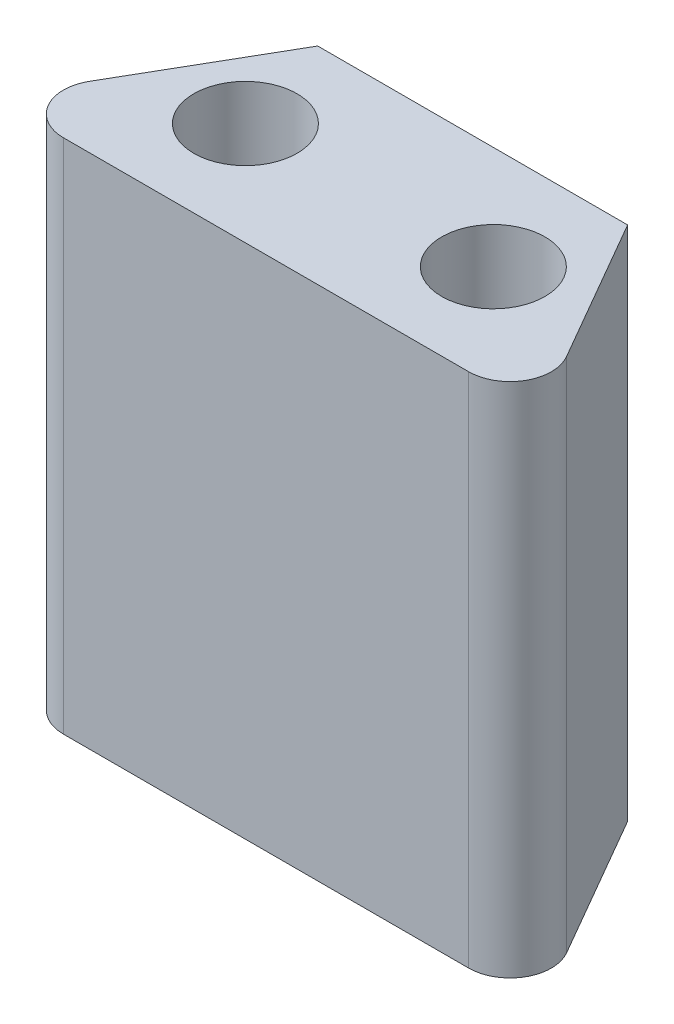
from build123d import *

# Parameters (mm, degrees)
BOSS_EXTRUDE1_DEPTH        = 12.5
SKETCH2_R                  = 2.5
CUT_EXTRUDE1_DEPTH         = 5
M3_TAPPED_HOLE1_D          = 2.5
M3_TAPPED_HOLE1_DEPTH      = 7.5
M3_TAPPED_HOLE1_TIP        = 0.751075774
F_3_2_3_2_DIAMETER_HOLE1_D = 3.2
SKETCH8_R                  = 3.3
CUT_EXTRUDE2_DEPTH         = 2


with BuildPart() as part:
    # Sketch1 → Boss-Extrude1 (new, symmetric)
    with BuildSketch(Plane(origin=(0, 0, 0), x_dir=(1, 0, 0), z_dir=(0, 1, 0))):
        with BuildLine():
            Line((3.464101615, 0), (23.082903769, 0))
            ThreePointArc((23.082903769, 0), (24.814954576, 1), (24.814954576, 3))
            Line((24.814954576, 3), (20.773502692, 10))
            Line((20.773502692, 10), (5.773502692, 10))
            Line((5.773502692, 10), (1.732050808, 3))
            ThreePointArc((1.732050808, 3), (1.732050808, 1), (3.464101615, 0))
        make_face()
    extrude(amount=BOSS_EXTRUDE1_DEPTH, both=True)

    # Sketch2 → Cut-Extrude1 (cut)
    with BuildSketch(Plane(origin=(0, 12.5, 0), x_dir=(1, 0, 0), z_dir=(0, 1, 0))):
        with Locations(Location((7.273502692, 5, 0), (0, 0, 270))):
            Circle(SKETCH2_R)
        with Locations(Location((19.273502692, 5, 0), (0, 0, 270))):
            Circle(SKETCH2_R)
    extrude(amount=-CUT_EXTRUDE1_DEPTH, mode=Mode.SUBTRACT)

    # M3 Tapped Hole1
    with Locations(Plane(origin=(0, 0, -10), x_dir=(-1, 0, 0), z_dir=(0, 0, -1))):
        with Locations((-13.273502692, -5), (-13.273502692, 5)):
            Hole(M3_TAPPED_HOLE1_D / 2, depth=M3_TAPPED_HOLE1_DEPTH)
            with Locations((0, 0, -(M3_TAPPED_HOLE1_DEPTH + M3_TAPPED_HOLE1_TIP / 2))):  # 118° drill point
                Cone(0, M3_TAPPED_HOLE1_D / 2, M3_TAPPED_HOLE1_TIP, mode=Mode.SUBTRACT)

    # Ø3.2 (3.2) Diameter Hole1 (through all)
    with Locations(Plane(origin=(0, 7.5, 0), x_dir=(-1, 0, 0), z_dir=(0, 1, 0))):
        with Locations((-19.273502692, -5), (-7.273502692, -5)):
            Hole(F_3_2_3_2_DIAMETER_HOLE1_D / 2)

    # Sketch8 → Cut-Extrude2 (cut)
    with BuildSketch(Plane.XZ.offset(12.5)):
        with Locations(Location((13.273502692, -5, 0), (0, 0, 270))):
            Circle(SKETCH8_R)
    extrude(amount=-CUT_EXTRUDE2_DEPTH, mode=Mode.SUBTRACT)


solid = part.part
